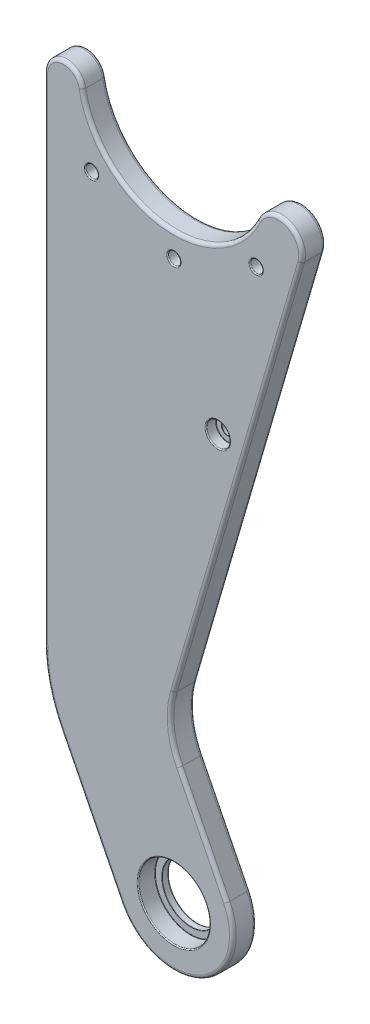
SolidWorks part; units mm, degrees
ref_plane "Front Plane" through (0, 0, 0) normal (0, 0, 1) x (1, 0, 0)
ref_plane "Top Plane" through (0, 0, 0) normal (0, 1, 0) x (1, 0, 0)
ref_plane "Right Plane" through (0, 0, 0) normal (1, 0, 0) x (0, 0, -1)
sketch "Sketch1" plane through (0, 0, 0) normal (0, 0, 1) x (1, 0, 0)
  line L2 (0, 0) -> (34.5, 0) construction
  line L3 (0, 0) -> (0, -200) construction
  line L4 (-38.4041, -5.7404) -> (-38.4041, -162.4687)
  line L5 (-38.4041, -162.4687) -> (-15.6424, -207.8463)
  line L6 (-30.7621, -72.1726) -> (-20.8155, -71.1406) construction
  line L7 (37.7376, -17.0663) -> (-2.7253, -155.5358)
  line L8 (-2.7253, -155.5358) -> (15.6424, -192.1537)
  arc A1 (-31.3715, -14.3555) -> (33.4286, -8.5309) centre (0, 0) ccw construction
  circle A5 centre (0, -34.5) radius 1.85
  circle A6 centre (24.3952, -24.3952) radius 1.85
  circle A7 centre (-24.3952, -24.3952) radius 1.85
  circle A10 centre (0, -200) radius 8.5
  arc A11 (-15.6424, -207.8463) -> (15.6424, -192.1537) centre (0, -200) ccw
  arc A20 (-27.0859, -4.7545) -> (24.7249, -12.0386) centre (0, 0) ccw
  arc A25 (-27.0859, -4.7545) -> (-38.4041, -5.7404) centre (-32.702, -5.7404) ccw
  arc A26 (37.7376, -17.0663) -> (24.7249, -12.0386) centre (31.0186, -15.1029) ccw
  point P28 (0, -100)
  dimension "D1" = 27.5
  dimension "D2" = 200
  dimension "D3" = 3.7
  dimension "D5" = 17
  dimension "D6" = 35
  dimension "D7" = 3.7
  dimension "D8" = 3.7
  dimension "D4" = 10
extrude "Boss-Extrude1" add sketch "Sketch1" along normal blind 7
sketch "Sketch2" plane through (0, 0, 7) normal (0, 0, 1) x (1, 0, 0)
  circle A0 centre (0, -200) radius 10.575
  dimension "D1" = 21.15
extrude "Cut-Extrude1" cut sketch "Sketch2" against normal blind 5
fillet "Fillet1" radius 25 1 edges at (-2.7253, -155.5358, 3.5)
fillet "Fillet2" radius 45 1 edges at (-38.4041, -162.4687, 3.5)
sketch "Sketch3" plane through (0, 0, 7) normal (0, 0, 1) x (1, 0, 0)
  line L0 (37.7376, -17.0663) -> (0.0317, -146.1008) construction
  circle A0 centre (13.0253, -73.1129) radius 1.85
  arc A1 (0.0317, -146.1008) -> (1.6819, -164.3219) centre (24.0282, -153.1129) ccw construction
  dimension "D1" = 3.7
  dimension "D2" = 8
  dimension "D3" = 80
extrude "Cut-Extrude2" cut sketch "Sketch3" against normal up to next
sketch "Sketch8" plane through (0, 0, 0) normal (0, 0, -1) x (-1, 0, 0)
  circle A0 centre (0, -34.5) radius 3.5
  circle A1 centre (-24.3952, -24.3952) radius 3.5
  circle A2 centre (24.3952, -24.3952) radius 3.5
  dimension "D1" = 7
  dimension "D2" = 7
  dimension "D3" = 7
extrude "Cut-Extrude7" cut sketch "Sketch8" against normal blind 3
sketch "Sketch9" plane through (0, 0, 7) normal (0, 0, 1) x (1, 0, 0)
  circle A0 centre (13.0253, -73.1129) radius 3.5
  dimension "D1" = 7
extrude "Cut-Extrude8" cut sketch "Sketch9" against normal blind 3
fillet "Fillet3" radius 1 20 edges at (33.5414, -8.5734, 7) (-3.8285, -27.2322, 7) (-33.1968, -0.0599, 7) (-38.4041, -78.7778, 7) (-37.1936, -162.1822, 7) (-24.6349, -189.9189, 7) (7.8463, -215.6424, 7) (8.6621, -178.2378, 7) (-0.8699, -155.3677, 7) (-33.1968, -0.0599, 0) (-3.8285, -27.2322, 0) (33.5414, -8.5734, 0) (18.8846, -81.5835, 0) (-0.8699, -155.3677, 0) (8.6621, -178.2378, 0) (7.8463, -215.6424, 0) (-24.6349, -189.9189, 0) (-37.1936, -162.1822, 0) (18.8846, -81.5835, 7) (-38.4041, -78.7778, 0)
fillet "Fillet4" radius 0.3 10 edges at (-22.5452, -24.3952, 7) (1.85, -34.5, 7) (26.2452, -24.3952, 7) (16.5253, -73.1129, 7) (20.8952, -24.3952, 0) (-27.8952, -24.3952, 0) (-3.5, -34.5, 0) (14.8753, -73.1129, 0) (8.5, -200, 0) (10.575, -200, 7)
fillet "Fillet5" radius 0.1 10 edges at (-26.2452, -24.3952, 3) (-27.8952, -24.3952, 3) (-1.85, -34.5, 3) (-3.5, -34.5, 3) (20.8952, -24.3952, 3) (22.5452, -24.3952, 3) (14.8753, -73.1129, 4) (16.5253, -73.1129, 4) (10.575, -200, 2) (8.5, -200, 2)
